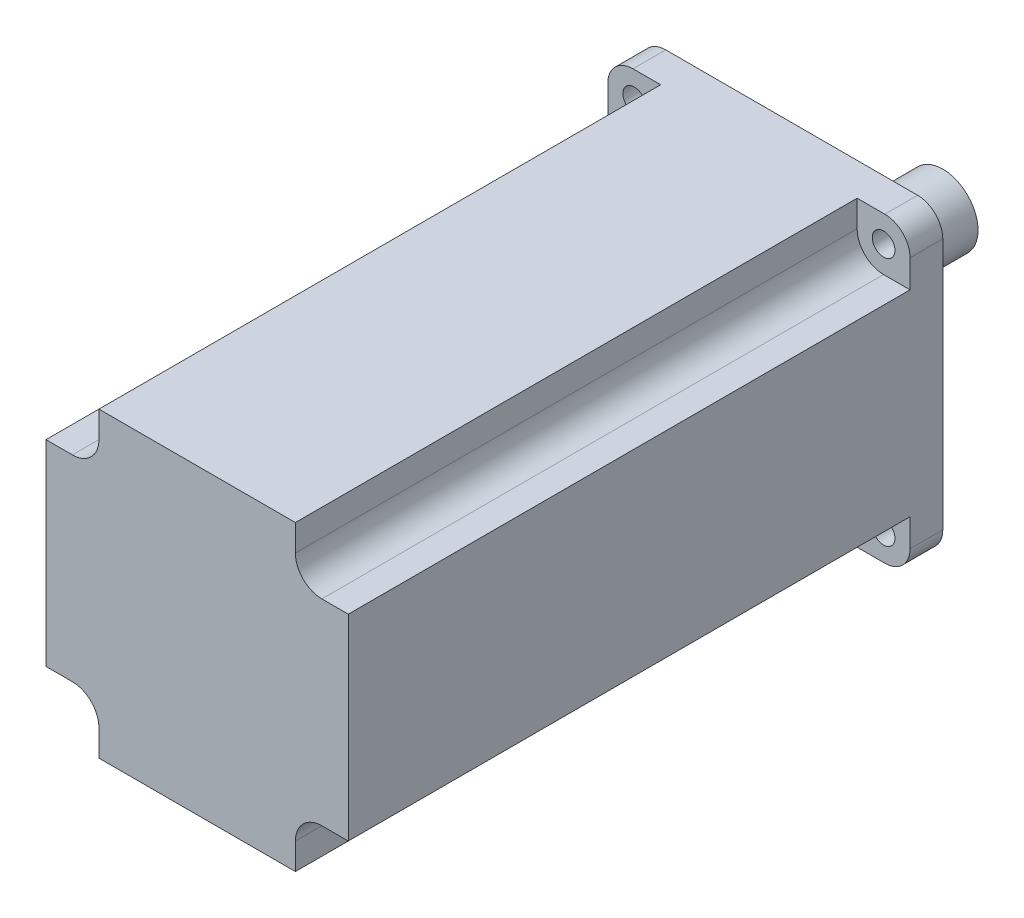
SolidWorks part; units mm, degrees
ref_plane "Front Plane" through (0, 0, 0) normal (0, 0, 1) x (1, 0, 0)
ref_plane "Top Plane" through (0, 0, 0) normal (0, 1, 0) x (1, 0, 0)
ref_plane "Right Plane" through (0, 0, 0) normal (1, 0, 0) x (0, 0, -1)
sketch "Sketch1" plane through (0, 0, 0) normal (0, 0, 1) x (1, 0, 0)
  line L0 (-24.7487, 24.7487) -> (24.7487, -24.7487) construction
  line L1 (-25, -30) -> (25, -30)
  line L2 (-30, -25) -> (-30, 25)
  line L3 (-25, 30) -> (25, 30)
  line L4 (30, -25) -> (30, 25)
  line L5 (24.7487, 24.7487) -> (-24.7487, -24.7487) construction
  line L6 (-35, 0) -> (35, 0) construction
  line L7 (0, 35) -> (0, -35) construction
  circle A0 centre (-24.7487, 24.7487) radius 2.25
  circle A1 centre (-24.7487, -24.7487) radius 2.25
  circle A2 centre (24.7487, -24.7487) radius 2.25
  circle A3 centre (24.7487, 24.7487) radius 2.25
  circle A4 centre (0, 0) radius 35 construction
  arc A5 (-30, 25) -> (-25, 30) centre (-25, 25) cw
  arc A6 (25, 30) -> (30, 25) centre (25, 25) cw
  arc A7 (25, -30) -> (30, -25) centre (25, -25) ccw
  arc A8 (-30, -25) -> (-25, -30) centre (-25, -25) ccw
  point P9 (-30, 30)
  point P24 (30, 30)
  point P29 (-30, -30)
  dimension "D8" = 70
  dimension "D5" = 4.5
  dimension "D9" = 5
  dimension "D1" = 60
  dimension "D2" = 60
  dimension "D3" = 30
  dimension "D4" = 30
  dimension "D6" = 45
  dimension "D7" = 45
extrude "Extrude1" add sketch "Sketch1" along normal blind 6.5
sketch "Sketch2" plane through (0, 0, 6.5) normal (0, 0, 1) x (1, 0, 0)
  line L1 (-19.4975, -30) -> (19.4975, -30)
  line L2 (-30, 19.4975) -> (-30, -19.4975)
  line L4 (30, 19.4975) -> (30, -19.4975)
  line L5 (-30, 25) -> (-30, -25) construction
  line L6 (30, -25) -> (30, 25) construction
  line L9 (-24.7487, 19.4975) -> (-30, 19.4975)
  line L10 (-19.4975, 24.7487) -> (-19.4975, 30)
  line L11 (19.4975, 24.7487) -> (19.4975, 30)
  line L12 (24.7487, 19.4975) -> (30, 19.4975)
  line L13 (24.7487, -19.4975) -> (30, -19.4975)
  line L14 (19.4975, -24.7487) -> (19.4975, -30)
  line L15 (-19.4975, -24.7487) -> (-19.4975, -30)
  line L16 (-24.7487, -19.4975) -> (-30, -19.4975)
  line L17 (-19.4975, 30) -> (19.4975, 30)
  arc A0 (-24.7487, 19.4975) -> (-19.4975, 24.7487) centre (-24.7487, 24.7487) ccw
  arc A1 (19.4975, 24.7487) -> (24.7487, 19.4975) centre (24.7487, 24.7487) ccw
  arc A2 (24.7487, -19.4975) -> (19.4975, -24.7487) centre (24.7487, -24.7487) ccw
  arc A3 (-19.4975, -24.7487) -> (-24.7487, -19.4975) centre (-24.7487, -24.7487) ccw
extrude "Extrude2" add sketch "Sketch2" along normal blind 111.5
sketch "Sketch3" plane through (0, 0, 0) normal (0, 0, -1) x (-1, 0, 0)
  circle A0 centre (0, 0) radius 25
  dimension "D1" = 50
extrude "Extrude3" add sketch "Sketch3" along normal blind 3
sketch "Sketch4" plane through (0, 0, -3) normal (0, 0, -1) x (-1, 0, 0)
  circle A0 centre (0, 0) radius 7
  dimension "D1" = 14
extrude "Extrude4" add sketch "Sketch4" along normal blind 27
